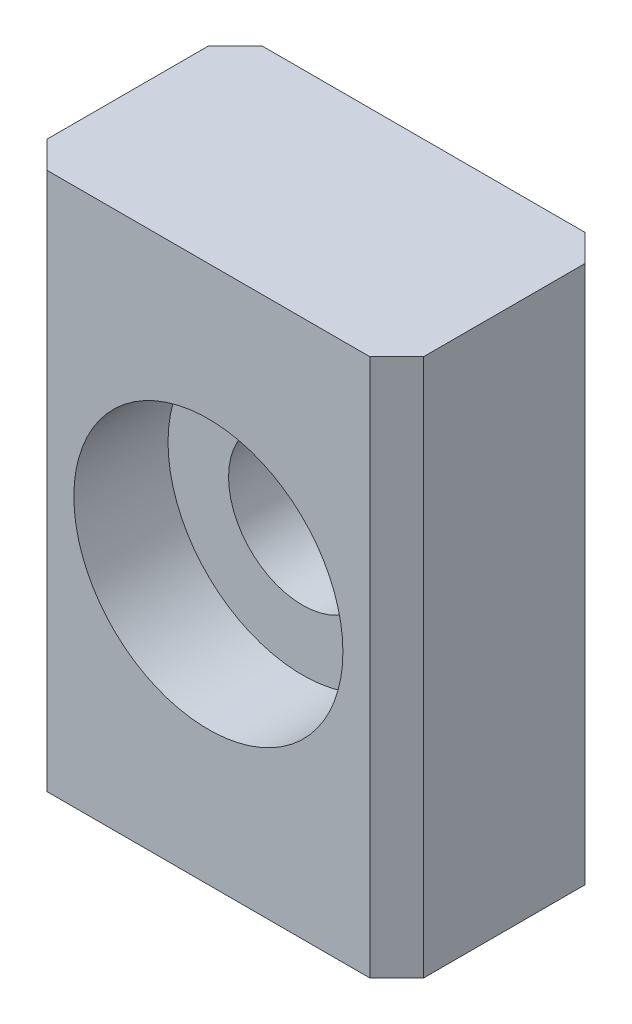
SolidWorks part; units mm, degrees
material "Nickel"
ref_plane "Front" through (0, 0, 0) normal (0, 0, 1) x (1, 0, 0)
ref_plane "Top" through (0, 0, 0) normal (0, 1, 0) x (1, 0, 0)
ref_plane "Right" through (0, 0, 0) normal (1, 0, 0) x (0, 0, -1)
sketch "Sketch1" plane through (0, 0, 0) normal (0, 0, 1) x (1, 0, 0)
  line L1 (0, 0) -> (-14, 0)
  line L2 (0, 0) -> (0, 20)
  line L3 (0, 20) -> (-14, 20)
  line L4 (-14, 0) -> (-14, 20)
  dimension "D1" = 20
  dimension "D2" = 14
extrude "Boss-Extrude" add sketch "Sketch1" against normal blind 8
sketch "Sketch2" plane through (0, 0, 0) normal (0, 0, 1) x (1, 0, 0)
  line L0 (-14, 10) -> (0, 10) construction
  line L1 (-14, 20) -> (-14, 0) construction
  line L2 (0, 0) -> (0, 20) construction
  line L3 (-7, 20) -> (-7, 0) construction
  line L4 (0, 20) -> (-14, 20) construction
  line L5 (-14, 0) -> (0, 0) construction
  circle A0 centre (-7, 10) radius 5
  dimension "D3" = 10
  dimension "D1" = 10
  dimension "D2" = 7
extrude "Cut-Extrude1" cut sketch "Sketch2" against normal blind 3.5
sketch "Sketch3" plane through (0, 0, -3.5) normal (0, 0, 1) x (1, 0, 0)
  circle A0 centre (-7, 10) radius 2.75
  dimension "D1" = 5.5
extrude "Cut-Extrude2" cut sketch "Sketch3" against normal through all
chamfer "Chamfer1" distance 1 angle 45 4 edges at (-14, 10, -8) (0, 10, -8) (-14, 10, 0) (0, 10, 0)
